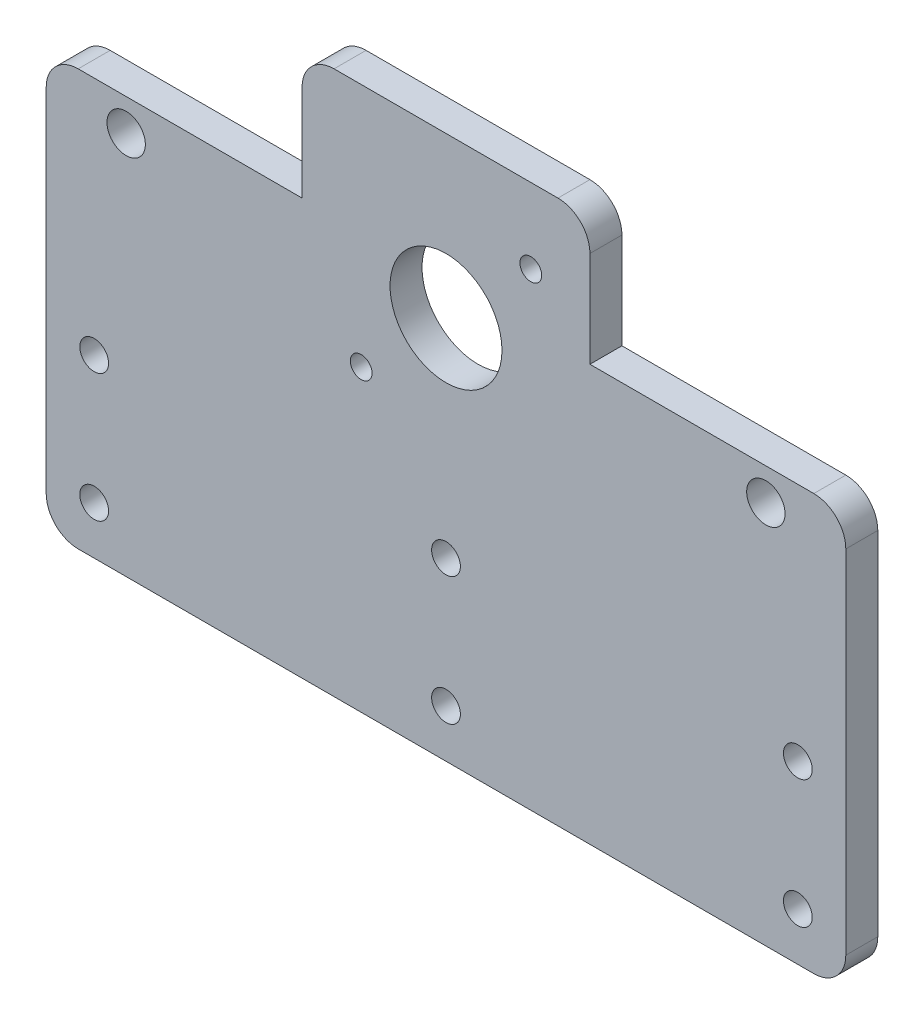
from build123d import *

# Parameters (mm, degrees)
SKETCH_1_W              = 250
SKETCH_1_H              = 170
EXTRUDE_1_DEPTH         = 5
SKETCH_2_W              = 80
SKETCH_2_H              = 40
CUT_EXTRUDE_1_DEPTH     = 10
HOLE_WIZARD_9_0_9_1_D   = 9
PATTERN_LINEAR_1_COUNT  = 3
PATTERN_LINEAR_1_PITCH  = 110
HOLE_WIZARD_12_0_12_1_D = 12
SKETCH_7_R              = 17.5
CUT_EXTRUDE_2_DEPTH     = 10
HOLE_WIZARD_M8_1_D      = 6.8
FILLET_1_R              = 10


with BuildPart() as part:
    # 草图1 → 凸台-拉伸1 (new, symmetric)
    with BuildSketch(Plane.XY):
        Rectangle(SKETCH_1_W, SKETCH_1_H)
    extrude(amount=EXTRUDE_1_DEPTH, both=True)

    # 草图2 → 切除-拉伸1 (cut)
    with BuildSketch(Plane.XY.offset(5)):
        with Locations((85, 65)):
            Rectangle(SKETCH_2_W, SKETCH_2_H)
    cut_extrude_1 = extrude(amount=-CUT_EXTRUDE_1_DEPTH, mode=Mode.SUBTRACT)

    # 镜向1: 切除-拉伸1 across plane
    add(cut_extrude_1.mirror(Plane(origin=(0, 0, 0), x_dir=(0, 0, 1), z_dir=(1, 0, 0))), mode=Mode.SUBTRACT)

    # Ø9.0 (9) 直径孔1 (through all)
    with Locations(Plane.XY.offset(5)):
        with Locations((-110, -30), (-110, -70)):
            hole_wizard_9_0_9_1 = Hole(HOLE_WIZARD_9_0_9_1_D / 2)

    # 阵列(线性)1: Ø9.0 (9) 直径孔1 ×3
    with Locations(*[(i * PATTERN_LINEAR_1_PITCH, 0, 0) for i in range(1, PATTERN_LINEAR_1_COUNT)]):
        add(hole_wizard_9_0_9_1, mode=Mode.SUBTRACT)

    # Ø12.0 (12) 直径孔1 (through all)
    with Locations(Plane.XY.offset(5)):
        with Locations((-100, 35), (100, 35)):
            Hole(HOLE_WIZARD_12_0_12_1_D / 2)

    # 草图7 → 切除-拉伸2 (cut)
    with BuildSketch(Plane.XY.offset(5)):
        with Locations((0, 35)):
            Circle(SKETCH_7_R)
    extrude(amount=-CUT_EXTRUDE_2_DEPTH, mode=Mode.SUBTRACT)

    # M8 螺纹孔1 (through all)
    with Locations(Plane.XY.offset(5)):
        with Locations((-26.515, 8.485), (26.515, 61.515)):
            Hole(HOLE_WIZARD_M8_1_D / 2)

    # 圆角1
    fillet_1_edges = [part.edges().sort_by_distance(p)[0] for p in [
        (45, 85, 0),
        (125, 45, 0),
        (-45, 85, 0),
        (-125, 45, 0),
        (125, -85, 0),
        (-125, -85, 0),
    ]]
    fillet(fillet_1_edges, radius=FILLET_1_R)


solid = part.part
